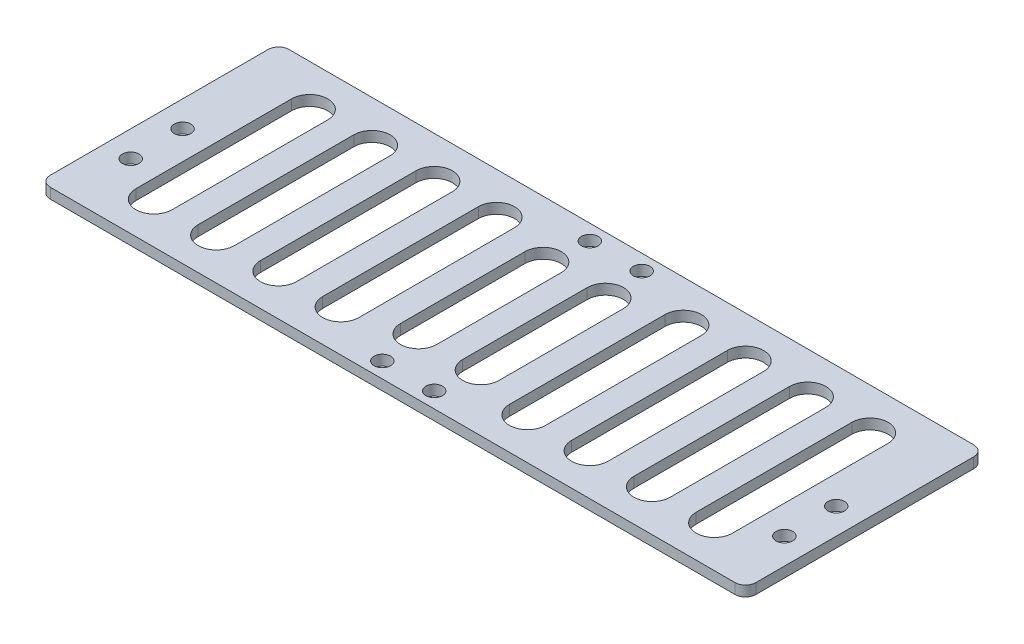
from build123d import *

# Parameters (mm, degrees)
SKETCH_1_W          = 136
SKETCH_1_H          = 46
SKETCH_1_R          = 1.6
EXTRUDE_1_DEPTH     = 2
CUT_EXTRUDE_1_DEPTH = 72.812255222
FILLET_R2_1_R       = 2


with BuildPart() as part:
    # 草图1 → 凸台-拉伸1 (new body)
    with BuildSketch(Plane(origin=(0, 0, 0), x_dir=(1, 0, 0), z_dir=(0, 1, 0))):
        Rectangle(SKETCH_1_W, SKETCH_1_H)
        with Locations(Location((-63, -0.5, 0), (0, 0, 270))):
            Circle(SKETCH_1_R, mode=Mode.SUBTRACT)
        with Locations(Location((-63, -10.5, 0), (0, 0, 270))):
            Circle(SKETCH_1_R, mode=Mode.SUBTRACT)
        with Locations(Location((-5, -20, 0), (0, 0, 270))):
            Circle(SKETCH_1_R, mode=Mode.SUBTRACT)
        with Locations(Location((5, -20, 0), (0, 0, 270))):
            Circle(SKETCH_1_R, mode=Mode.SUBTRACT)
        with Locations(Location((63, -10.5, 0), (0, 0, 90))):
            Circle(SKETCH_1_R, mode=Mode.SUBTRACT)
        with Locations(Location((63, -0.5, 0), (0, 0, 90))):
            Circle(SKETCH_1_R, mode=Mode.SUBTRACT)
        with Locations(Location((5, 20, 0), (0, 0, 90))):
            Circle(SKETCH_1_R, mode=Mode.SUBTRACT)
        with Locations(Location((-5, 20, 0), (0, 0, 90))):
            Circle(SKETCH_1_R, mode=Mode.SUBTRACT)
    extrude(amount=EXTRUDE_1_DEPTH)

    # 草图2 → 切除-拉伸1 (cut, through all)
    with BuildSketch(Plane(origin=(0, 2, 0), x_dir=(1, 0, 0), z_dir=(0, 1, 0))):
        with BuildLine():
            Line((-50.5, 15), (-50.5, -15))
            ThreePointArc((-50.5, -15), (-54, -18.5), (-57.5, -15))
            Line((-57.5, -15), (-57.5, 15))
            ThreePointArc((-57.5, 15), (-54, 18.5), (-50.5, 15))
        make_face()
        with BuildLine():
            Line((-38.5, 15), (-38.5, -15))
            ThreePointArc((-38.5, -15), (-42, -18.5), (-45.5, -15))
            Line((-45.5, -15), (-45.5, 15))
            ThreePointArc((-45.5, 15), (-42, 18.5), (-38.5, 15))
        make_face()
        with BuildLine():
            Line((-26.5, 15), (-26.5, -15))
            ThreePointArc((-26.5, -15), (-30, -18.5), (-33.5, -15))
            Line((-33.5, -15), (-33.5, 15))
            ThreePointArc((-33.5, 15), (-30, 18.5), (-26.5, 15))
        make_face()
        with BuildLine():
            Line((-14.5, 15), (-14.5, -15))
            ThreePointArc((-14.5, -15), (-18, -18.5), (-21.5, -15))
            Line((-21.5, -15), (-21.5, 15))
            ThreePointArc((-21.5, 15), (-18, 18.5), (-14.5, 15))
        make_face()
        with BuildLine():
            Line((-2.5, 12), (-2.5, -12))
            ThreePointArc((-2.5, -12), (-6, -15.5), (-9.5, -12))
            Line((-9.5, -12), (-9.5, 12))
            ThreePointArc((-9.5, 12), (-6, 15.5), (-2.5, 12))
        make_face()
        with BuildLine():
            Line((9.5, 12), (9.5, -12))
            ThreePointArc((9.5, -12), (6, -15.5), (2.5, -12))
            Line((2.5, -12), (2.5, 12))
            ThreePointArc((2.5, 12), (6, 15.5), (9.5, 12))
        make_face()
        with BuildLine():
            Line((21.5, 15), (21.5, -15))
            ThreePointArc((21.5, -15), (18, -18.5), (14.5, -15))
            Line((14.5, -15), (14.5, 15))
            ThreePointArc((14.5, 15), (18, 18.5), (21.5, 15))
        make_face()
        with BuildLine():
            Line((33.5, 15), (33.5, -15))
            ThreePointArc((33.5, -15), (30, -18.5), (26.5, -15))
            Line((26.5, -15), (26.5, 15))
            ThreePointArc((26.5, 15), (30, 18.5), (33.5, 15))
        make_face()
        with BuildLine():
            Line((45.5, 15), (45.5, -15))
            ThreePointArc((45.5, -15), (42, -18.5), (38.5, -15))
            Line((38.5, -15), (38.5, 15))
            ThreePointArc((38.5, 15), (42, 18.5), (45.5, 15))
        make_face()
        with BuildLine():
            Line((57.5, 15), (57.5, -15))
            ThreePointArc((57.5, -15), (54, -18.5), (50.5, -15))
            Line((50.5, -15), (50.5, 15))
            ThreePointArc((50.5, 15), (54, 18.5), (57.5, 15))
        make_face()
    extrude(amount=-CUT_EXTRUDE_1_DEPTH, mode=Mode.SUBTRACT)

    # R2 圆角1
    fillet_r2_1_edges = [part.edges().sort_by_distance(p)[0] for p in [
        (-68, 1, -23),
        (68, 1, -23),
        (68, 1, 23),
        (-68, 1, 23),
    ]]
    fillet(fillet_r2_1_edges, radius=FILLET_R2_1_R)


solid = part.part
